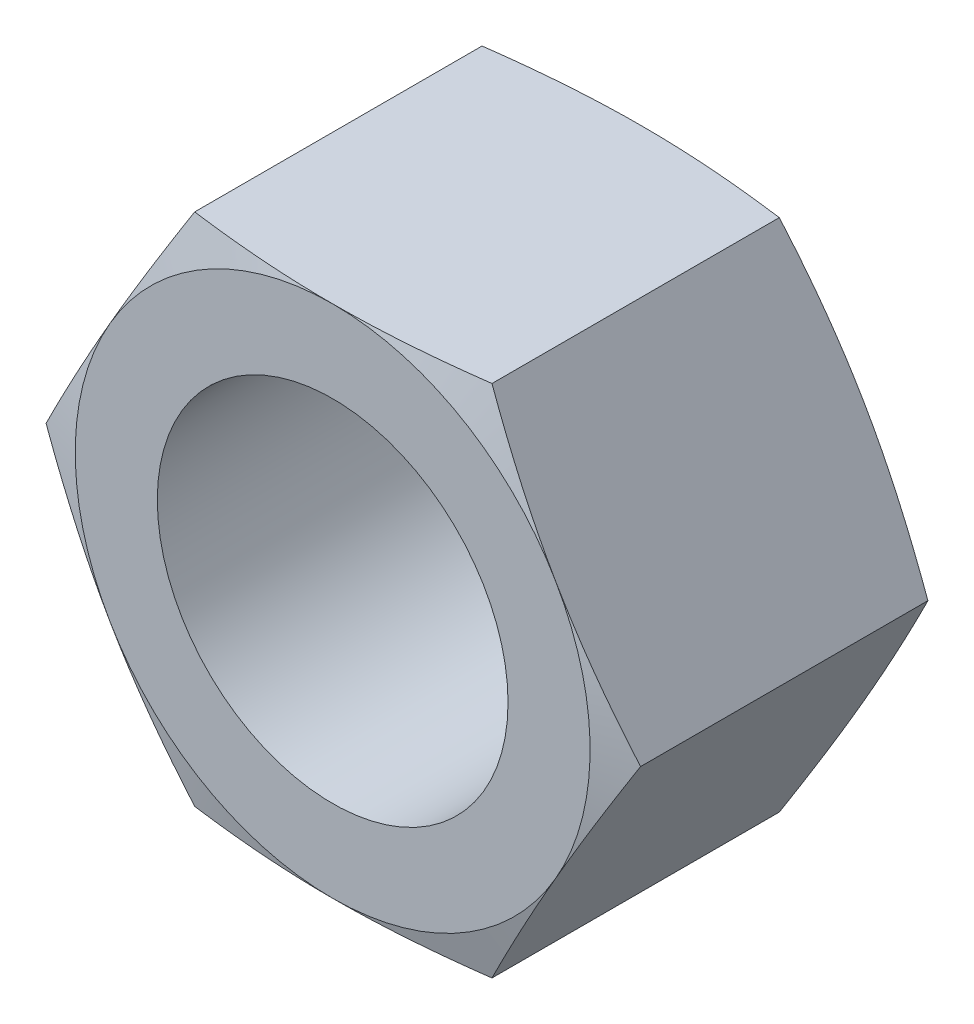
from build123d import *

# Parameters (mm, degrees)
SKETCH_1_R          = 15
EXTRUDE_519_DEPTH   = 26.4
SKETCH_2_OUTSIDE_W  = 350.938
SKETCH_2_OUTSIDE_H  = 344.126
SKETCH_2_OUTSIDE_R  = 22.018695891
CUT_EXTRUDE_1_DEPTH = 38
CUT_EXTRUDE_1_DRAFT = -75
SKETCH_3_OUTSIDE_W  = 350.938
SKETCH_3_OUTSIDE_H  = 344.126
SKETCH_3_OUTSIDE_R  = 22.018695891
CUT_EXTRUDE_2_DEPTH = 38
CUT_EXTRUDE_2_DRAFT = -75


with BuildPart() as part:
    # 草图1 → Extrude 519 (new body)
    with BuildSketch(Plane.XY):
        Polygon((12.7125, 22.018695891), (-12.7125, 22.018695891), (-25.425, 0), (-12.7125, -22.018695891), (12.7125, -22.018695891), (25.425, 0), align=None)
        Circle(SKETCH_1_R, mode=Mode.SUBTRACT)
    extrude(amount=EXTRUDE_519_DEPTH)


with BuildPart() as cut_extrude_1_tool:
    # 草图2 outside → 切除-拉伸1 (with draft: the straight prism first)
    with BuildSketch(Plane(origin=(0, 0, 0), x_dir=(-1, 0, 0), z_dir=(0, 0, -1))):
        Rectangle(SKETCH_2_OUTSIDE_W, SKETCH_2_OUTSIDE_H)
        Circle(SKETCH_2_OUTSIDE_R, mode=Mode.SUBTRACT)
    extrude(amount=-CUT_EXTRUDE_1_DEPTH)
    # 切除-拉伸1: the draft: its side faces are tilted about the plane it starts from
    cut_extrude_1_sides = [cut_extrude_1_tool.faces().sort_by_distance(p)[0] for p in [
        (0, -172.063, 19),
        (-175.469, 0, 19),
        (0, 172.063, 19),
        (175.469, 0, 19),
        (22.018695891, 0, 19),
    ]]
    draft(cut_extrude_1_sides, Plane(origin=(0, 0, 0), x_dir=(-1, 0, 0), z_dir=(0, 0, -1)), CUT_EXTRUDE_1_DRAFT)


with BuildPart() as part_1:
    add(part.part)

    # 切除-拉伸1: cut by cut_extrude_1_tool
    add(cut_extrude_1_tool.part, mode=Mode.SUBTRACT)


with BuildPart() as cut_extrude_2_tool:
    # 草图3 outside → 切除-拉伸2 (with draft: the straight prism first)
    with BuildSketch(Plane.XY.offset(26.4)):
        Rectangle(SKETCH_3_OUTSIDE_W, SKETCH_3_OUTSIDE_H)
        Circle(SKETCH_3_OUTSIDE_R, mode=Mode.SUBTRACT)
    extrude(amount=-CUT_EXTRUDE_2_DEPTH)
    # 切除-拉伸2: the draft: its side faces are tilted about the plane it starts from
    cut_extrude_2_sides = [cut_extrude_2_tool.faces().sort_by_distance(p)[0] for p in [
        (0, -172.063, 7.4),
        (175.469, 0, 7.4),
        (0, 172.063, 7.4),
        (-175.469, 0, 7.4),
        (-22.018695891, 0, 7.4),
    ]]
    draft(cut_extrude_2_sides, Plane.XY.offset(26.4), CUT_EXTRUDE_2_DRAFT)


with BuildPart() as part_2:
    add(part_1.part)

    # 切除-拉伸2: cut by cut_extrude_2_tool
    add(cut_extrude_2_tool.part, mode=Mode.SUBTRACT)


solid = part_2.part
